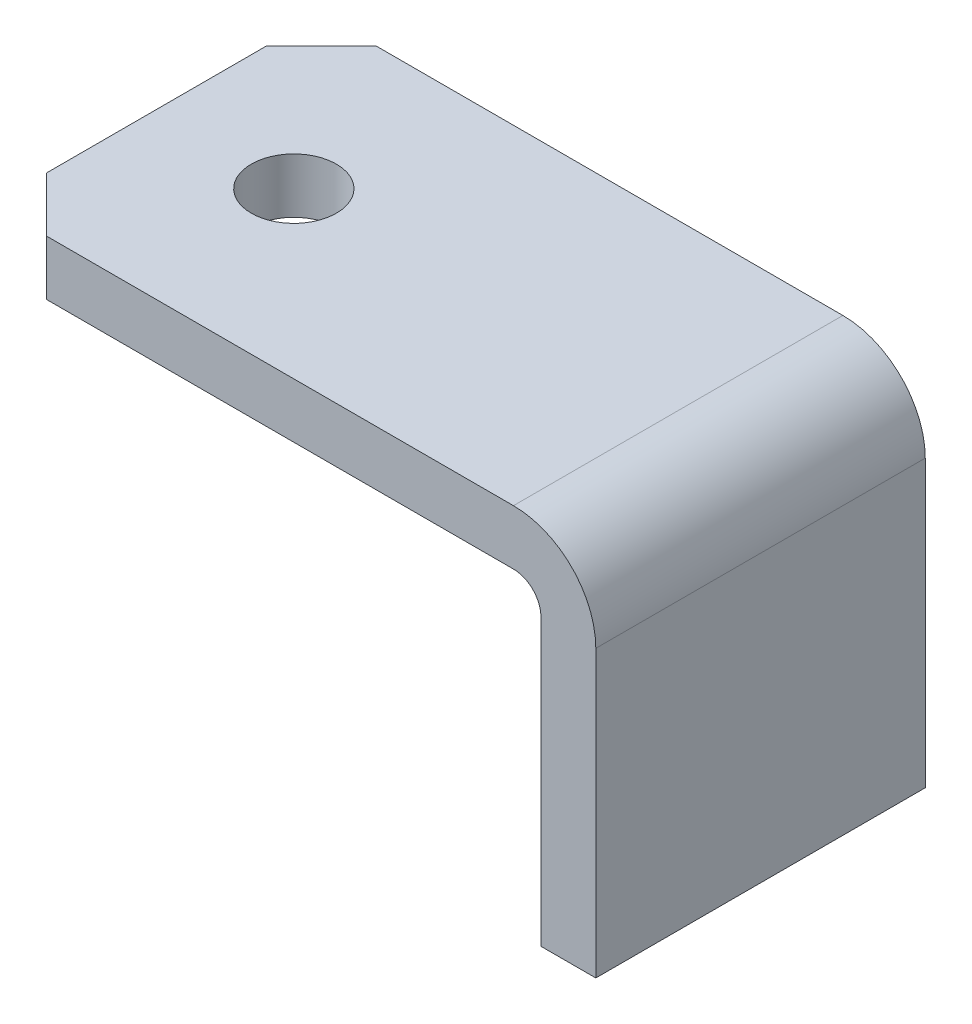
SolidWorks part; units mm, degrees
material "1023 碳钢板 (SS)"
ref_plane "Front Plane" through (0, 0, 0) normal (0, 0, 1) x (1, 0, 0)
ref_plane "Top Plane" through (0, 0, 0) normal (0, 1, 0) x (1, 0, 0)
ref_plane "Right Plane" through (0, 0, 0) normal (1, 0, 0) x (0, 0, -1)
sketch "Sketch1" plane through (0, 0, 0) normal (0, 0, 1) x (1, 0, 0)
  line L0 (0, 0) -> (95, 0)
  line L1 (110, -15) -> (110, -67)
  line L2 (0, -10) -> (95, -10)
  line L3 (100, -15) -> (100, -67)
  line L4 (0, -10) -> (0, 0)
  line L5 (110, -67) -> (100, -67)
  arc A0 (95, 0) -> (110, -15) centre (95, -15) cw
  arc A1 (95, -10) -> (100, -15) centre (95, -15) cw
  point P6 (110, 0)
  dimension "D3" = 15
  dimension "D1" = 110
  dimension "D2" = 67
  dimension "D4" = 10
extrude "Boss-Extrude1" add sketch "Sketch1" along normal blind 60
chamfer "Chamfer1" distance 10 angle 45 2 edges at (0, -5, 0) (0, -5, 60)
sketch "Sketch2" plane through (0, 0, 0) normal (0, 1, 0) x (1, 0, 0)
  line L0 (0, -50) -> (0, -10) construction
  circle A0 centre (25, -30) radius 5.1111
  dimension "D1" = 25
hole_wizard "M18 Tapped Hole1" positions "Sketch3" profile "Sketch4" tap size "M18" standard "ISO"
sketch "Sketch3" plane through (0, 0, 0) normal (0, 1, 0) x (1, 0, 0)
  point P0 (25, -30)
sketch "Sketch4" plane through (25, 0, 30) normal (1, 0, 0) x (0, 0, 1)
  line L0 (0, 0) -> (0, 48.1567)
  line L1 (0, 48.1567) -> (7.75, 43.5)
  line L2 (7.75, 43.5) -> (7.75, 0)
  line L5 (7.75, 0) -> (0, 0)
  line L10 (0, 48.1567) -> (-7.75, 43.5) construction
  line L11 (0, -6.35) -> (0, 107.95) construction
  dimension "螺纹孔钻头直径" = 15.5
  dimension "螺纹孔钻头深度" = 43.5
  dimension "导头角度" = 118
cosmetic thread "Hole Thread Line1" parameters "D1"=36, "D2"=18
